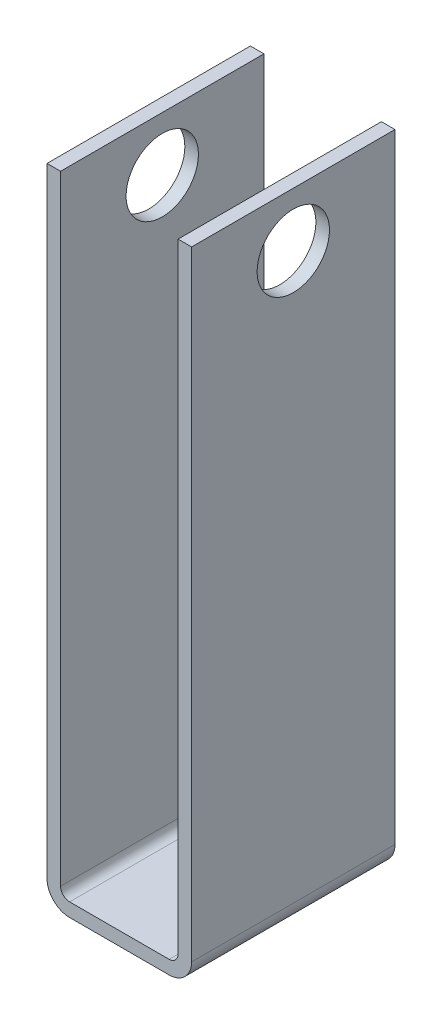
from build123d import *

# Parameters (mm, degrees)
BOSS_EXTRUDE1_DEPTH = 45
SKETCH2_R           = 8
CUT_EXTRUDE1_DEPTH  = 153.358130732


with BuildPart() as part:
    # Sketch1 → Boss-Extrude1 (new body)
    with BuildSketch(Plane.XY):
        with BuildLine():
            Line((0, 0), (0, -137))
            ThreePointArc((0, -137), (1.464466094, -140.535533906), (5, -142))
            Line((5, -142), (27, -142))
            ThreePointArc((27, -142), (30.535533906, -140.535533906), (32, -137))
            Line((32, -137), (32, 0))
            Line((32, 0), (29, 0))
            Line((29, 0), (29, -137))
            ThreePointArc((29, -137), (28.414213562, -138.414213562), (27, -139))
            Line((27, -139), (5, -139))
            ThreePointArc((5, -139), (3.585786438, -138.414213562), (3, -137))
            Line((3, -137), (3, 0))
            Line((3, 0), (0, 0))
        make_face()
    extrude(amount=BOSS_EXTRUDE1_DEPTH)

    # Sketch2 → Cut-Extrude1 (cut, through all)
    with BuildSketch(Plane(origin=(32, 0, 0), x_dir=(0, 0, -1), z_dir=(1, 0, 0))):
        with Locations((-22.5, -12)):
            Circle(SKETCH2_R)
    extrude(amount=-CUT_EXTRUDE1_DEPTH, mode=Mode.SUBTRACT)


solid = part.part
